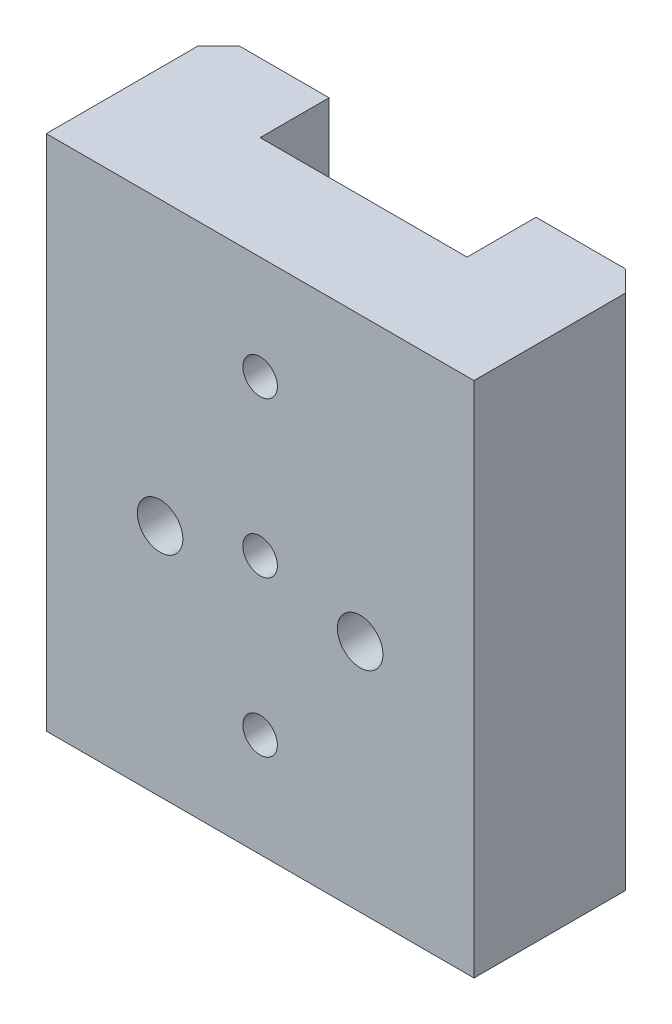
SolidWorks part; units mm, degrees
ref_plane "前视基准面" through (0, 0, 0) normal (0, 0, 1) x (1, 0, 0)
ref_plane "上视基准面" through (0, 0, 0) normal (0, 1, 0) x (1, 0, 0)
ref_plane "右视基准面" through (0, 0, 0) normal (1, 0, 0) x (0, 0, -1)
sketch "草图1" plane through (0, 0, 0) normal (0, 0, 1) x (1, 0, 0)
  line L1 (-31, 37.5) -> (31, 37.5)
  line L2 (-31, 37.5) -> (-31, -37.5)
  line L3 (-31, -37.5) -> (31, -37.5)
  line L4 (31, 37.5) -> (31, -37.5)
  line L5 (-31, 37.5) -> (31, -37.5) construction
  line L6 (-31, -37.5) -> (31, 37.5) construction
  point P0 (0, 0)
  dimension "D1" = 62
  dimension "D2" = 75
extrude "凸台-拉伸1" add sketch "草图1" along normal mid plane 25
hole_wizard "M6 螺纹孔1" positions "草图7" profile "草图6" tap size "M6" standard "ISO" end condition through all
sketch "草图7" plane through (0, 0, 12.5) normal (0, 0, 1) x (1, 0, 0)
  point P2 (0, 0)
sketch "草图6" plane through (0, 0, 12.5) normal (1, 0, 0) x (0, -1, 0)
  line L0 (0, 0) -> (0, 25)
  line L1 (0, 25) -> (2.5, 25)
  line L2 (2.5, 25) -> (2.5, 0)
  line L5 (2.5, 0) -> (0, 0)
  line L11 (0, -6.35) -> (0, 107.95) construction
  dimension "通孔螺纹孔钻头直径" = 5
  dimension "通孔螺纹孔钻头深度" = 25
cosmetic thread "孔螺蚊线2" parameters "D2"=6
chamfer "倒角1" distance 3 angle 45 2 edges at (31, 0, -12.5) (-31, 0, -12.5)
sketch "草图8" plane through (0, 0, -12.5) normal (0, 0, -1) x (-1, 0, 0)
  line L0 (-28, 37.5) -> (28, 37.5) construction
  line L2 (-15, 37.5) -> (15, 37.5)
  line L4 (-15, 37.5) -> (-15, -37.5)
  line L5 (-15, -37.5) -> (15, -37.5)
  line L6 (15, 37.5) -> (15, -37.5)
  line L7 (28, -37.5) -> (-28, -37.5) construction
  line L8 (0, 37.5) -> (0, -70.6512) construction
  dimension "D1" = 30
extrude "切除-拉伸1" cut sketch "草图8" against normal blind 10
hole_wizard "M6 螺纹孔2" positions "草图10" profile "草图9" tap size "M6" standard "ISO" end condition through all
sketch "草图10" plane through (0, 0, -2.5) normal (0, 0, -1) x (-1, 0, 0)
  point P15 (0, 22.5)
  point P18 (0, -22.5)
sketch "草图9" plane through (0, 22.5, -2.5) normal (1, 0, 0) x (0, 1, 0)
  line L0 (0, 0) -> (0, 15)
  line L1 (0, 15) -> (2.5, 15)
  line L2 (2.5, 15) -> (2.5, 0)
  line L5 (2.5, 0) -> (0, 0)
  line L11 (0, -6.35) -> (0, 107.95) construction
  dimension "通孔螺纹孔钻头直径" = 5
  dimension "通孔螺纹孔钻头深度" = 15
cosmetic thread "孔螺蚊线3" parameters "D2"=6
cosmetic thread "孔螺蚊线4" parameters "D2"=6
hole_wizard "M6 六角凹头螺钉的柱形沉头孔1" positions "草图12" profile "草图11" counterbore size "M6" standard "ISO" end condition through all
sketch "草图12" plane through (0, 0, -12.5) normal (0, 0, -1) x (-1, 0, 0)
  point P0 (-14.5, -3.5)
  point P3 (14.5, -3.5)
sketch "草图11" plane through (14.5, -3.5, -12.5) normal (1, 0, 0) x (0, 1, 0)
  line L0 (0, 0) -> (0, 25)
  line L1 (0, 25) -> (3.3, 25)
  line L3 (3.3, 25) -> (3.3, 20)
  line L4 (3.3, 20) -> (5.5, 20)
  line L5 (5.5, 20) -> (5.5, 0)
  line L7 (5.5, 0) -> (0, 0)
  line L11 (0, -6.35) -> (0, 107.95) construction
  dimension "通孔孔直径" = 6.6
  dimension "通孔孔深度" = 25
  dimension "柱形沉头孔直径" = 11
  dimension "柱形沉头孔深度" = 20
